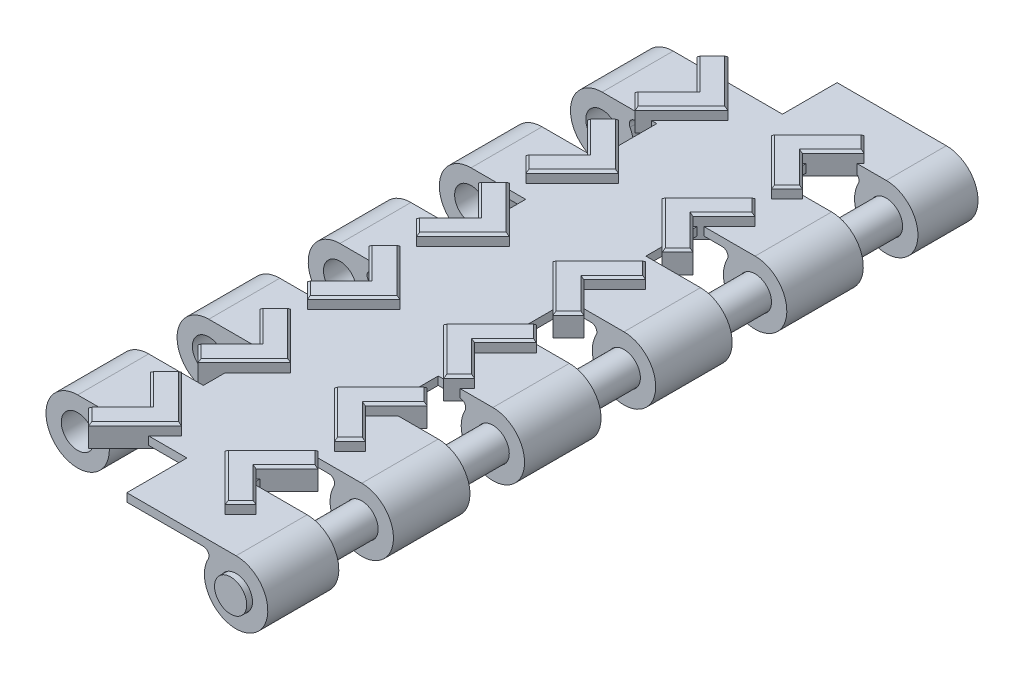
from build123d import *

# Parameters (mm, degrees)
BOSS_EXTRUDE1_DEPTH = 65
SKETCH2_W           = 12.9
SKETCH2_H           = 5.5
SKETCH2_H_2         = 5
CUT_EXTRUDE1_DEPTH  = 78.518380207
BOSS_EXTRUDE2_START = 5
SKETCH3_6_W         = 5
SKETCH3_6_H         = 0.75
BOSS_EXTRUDE2_DEPTH = 48
BOSS_EXTRUDE3_START = 32.5
BOSS_EXTRUDE3_DEPTH = 7.5
SKETCH6_R           = 1.5
CUT_EXTRUDE2_DEPTH  = 78.518380207
BOSS_EXTRUDE5_REACH = 79.518
SKETCH_3_6_W        = 5
SKETCH_3_6_H        = 0.75
SKETCH10_R          = 1.475
BOSS_EXTRUDE6_DEPTH = 33
BOSS_EXTRUDE9_DEPTH = 1
CHAMFER3_SIZE       = 0.2


with BuildPart() as part:
    # Sketch1 → Boss-Extrude1 (new body)
    with BuildSketch(Plane.XY):
        with BuildLine():
            Line((10, 40.220508076), (-10, 40.220508076))
            ThreePointArc((-10, 40.220508076), (-12.511473671, 38.770508076), (-12.511473671, 35.870508076))
            Line((-12.511473671, 35.870508076), (-10, 37.320508076))
            Line((-10, 37.320508076), (-7.1, 37.320508076))
            ThreePointArc((-7.1, 37.320508076), (-7.189694081, 38.036176043), (-7.453228027, 38.70757423))
            ThreePointArc((-7.453228027, 38.70757423), (-7.443701391, 39.218003951), (-7, 39.470508076))
            Line((-7, 39.470508076), (7, 39.470508076))
            ThreePointArc((7, 39.470508076), (7.443701391, 39.218003951), (7.453228027, 38.70757423))
            ThreePointArc((7.453228027, 38.70757423), (7.189694081, 38.036176043), (7.1, 37.320508076))
            Line((7.1, 37.320508076), (10, 37.320508076))
            Line((10, 37.320508076), (12.511473671, 35.870508076))
            ThreePointArc((12.511473671, 35.870508076), (12.511473671, 38.770508076), (10, 40.220508076))
        make_face()
        with BuildLine():
            ThreePointArc((7.1, 37.320508076), (9.249424769, 34.519323179), (12.511473671, 35.870508076))
            Line((12.511473671, 35.870508076), (10, 37.320508076))
            Line((10, 37.320508076), (7.1, 37.320508076))
        make_face()
        with BuildLine():
            Line((-10, 37.320508076), (-12.511473671, 35.870508076))
            ThreePointArc((-12.511473671, 35.870508076), (-9.249424769, 34.519323179), (-7.1, 37.320508076))
            Line((-7.1, 37.320508076), (-10, 37.320508076))
        make_face()
    extrude(amount=BOSS_EXTRUDE1_DEPTH)

    # Sketch2 → Cut-Extrude1 (cut, through all)
    with BuildSketch(Plane(origin=(0, 0, 0), x_dir=(1, 0, 0), z_dir=(0, 1, 0))):
        with Locations((-6.45, -50.25)):
            Rectangle(SKETCH2_W, SKETCH2_H)
        with Locations((-6.45, -62.25)):
            Rectangle(SKETCH2_W, SKETCH2_H)
        with Locations((-6.45, -38.25)):
            Rectangle(SKETCH2_W, SKETCH2_H)
        with Locations((-6.45, -26.25)):
            Rectangle(SKETCH2_W, SKETCH2_H)
        with Locations((-6.45, -14.25)):
            Rectangle(SKETCH2_W, SKETCH2_H)
        with Locations((-6.45, -2.25)):
            Rectangle(SKETCH2_W, SKETCH2_H)
        with Locations((6.45, -44)):
            Rectangle(SKETCH2_W, SKETCH2_H_2)
        with Locations((6.45, -56)):
            Rectangle(SKETCH2_W, SKETCH2_H_2)
        with Locations((6.45, -32)):
            Rectangle(SKETCH2_W, SKETCH2_H_2)
        with Locations((6.45, -20)):
            Rectangle(SKETCH2_W, SKETCH2_H_2)
        with Locations((6.45, -8)):
            Rectangle(SKETCH2_W, SKETCH2_H_2)
    extrude(amount=CUT_EXTRUDE1_DEPTH, mode=Mode.SUBTRACT)

    # Sketch3<6> → Boss-Extrude2 (add)
    with BuildSketch(Plane.XY.offset(BOSS_EXTRUDE2_START)):
        with Locations((-2.5, 39.845508076)):
            Rectangle(SKETCH3_6_W, SKETCH3_6_H)
    extrude(amount=BOSS_EXTRUDE2_DEPTH)

    # Sketch5 → Boss-Extrude3 (add, symmetric)
    with BuildSketch(Plane.XY.offset(BOSS_EXTRUDE3_START)):
        Polygon((-4, 39.470508076), (4, 39.470508076), (1.5, 36.470508076), (-1.5, 36.470508076), align=None)
    extrude(amount=BOSS_EXTRUDE3_DEPTH, both=True)

    # Sketch6 → Cut-Extrude2 (cut, through all)
    with BuildSketch(Plane(origin=(0, 0, 0), x_dir=(-1, 0, 0), z_dir=(0, 0, -1))):
        with Locations((-10, 37.320508076)):
            Circle(SKETCH6_R)
        with Locations((10, 37.320508076)):
            Circle(SKETCH6_R)
    extrude(amount=-CUT_EXTRUDE2_DEPTH, mode=Mode.SUBTRACT)

    # Boss-Extrude5: up to this face of the body (flat: up to its plane)
    boss_extrude5_end = Plane(part.part.faces().sort_by_distance((8.570145796, 37.969067426, 58.5))[0])
    # 草图3<6> → Boss-Extrude5 (add, up to the picked face)
    with BuildSketch(Plane.XY, mode=Mode.PRIVATE) as boss_extrude5_sk1:
        with Locations((2.5, 39.845508076)):
            Rectangle(SKETCH_3_6_W, SKETCH_3_6_H)
    boss_extrude5_tool1 = split(extrude(boss_extrude5_sk1.sketch, amount=BOSS_EXTRUDE5_REACH, mode=Mode.PRIVATE), bisect_by=boss_extrude5_end, keep=Keep.BOTH, mode=Mode.PRIVATE)
    add(boss_extrude5_tool1.solids().sort_by(Axis((2.5, 39.845508, 0), (0, 0, 1)))[0])

    # Sketch12 → Boss-Extrude9 (add, symmetric)
    with BuildSketch(Plane(origin=(0, 40.220508076, 0), x_dir=(1, 0, 0), z_dir=(0, 1, 0))):
        Polygon((-6.242640687, -3.757359313), (-2, -8), (-6.242640687, -12.242640687), (-7.656854249, -10.828427125), (-4.828427125, -8), (-7.656854249, -5.171572875), align=None)
        Polygon((-6.242640687, -13.757359313), (-2, -18), (-6.242640687, -22.242640687), (-7.656854249, -20.828427125), (-4.828427125, -18), (-7.656854249, -15.171572875), align=None)
        Polygon((-6.242640687, -23.757359313), (-2, -28), (-6.242640687, -32.242640687), (-7.656854249, -30.828427125), (-4.828427125, -28), (-7.656854249, -25.171572875), align=None)
        Polygon((-6.242640687, -33.757359313), (-2, -38), (-6.242640687, -42.242640687), (-7.656854249, -40.828427125), (-4.828427125, -38), (-7.656854249, -35.171572875), align=None)
        Polygon((-6.242640687, -43.757359313), (-2, -48), (-6.242640687, -52.242640687), (-7.656854249, -50.828427125), (-4.828427125, -48), (-7.656854249, -45.171572875), align=None)
        Polygon((-6.242640687, -53.757359313), (-2, -58), (-6.242640687, -62.242640687), (-7.656854249, -60.828427125), (-4.828427125, -58), (-7.656854249, -55.171572875), align=None)
        Polygon((4.828427125, -58), (7.656854249, -55.171572875), (6.242640687, -53.757359313), (2, -58), (6.242640687, -62.242640687), (7.656854249, -60.828427125), align=None)
        Polygon((2, -48), (6.242640687, -52.242640687), (7.656854249, -50.828427125), (4.828427125, -48), (7.656854249, -45.171572875), (6.242640687, -43.757359313), align=None)
        Polygon((2, -38), (6.242640687, -42.242640687), (7.656854249, -40.828427125), (4.828427125, -38), (7.656854249, -35.171572875), (6.242640687, -33.757359313), align=None)
        Polygon((2, -28), (6.242640687, -32.242640687), (7.656854249, -30.828427125), (4.828427125, -28), (7.656854249, -25.171572875), (6.242640687, -23.757359313), align=None)
        Polygon((7.656854249, -20.828427125), (4.828427125, -18), (7.656854249, -15.171572875), (6.242640687, -13.757359313), (2, -18), (6.242640687, -22.242640687), align=None)
        Polygon((7.656854249, -5.171572875), (6.242640687, -3.757359313), (2, -8), (6.242640687, -12.242640687), (7.656854249, -10.828427125), (4.828427125, -8), align=None)
    extrude(amount=BOSS_EXTRUDE9_DEPTH, both=True)

    # Chamfer3
    chamfer3_edges = [part.edges().sort_by_distance(p)[0] for p in [
        (4.121320344, 41.220508076, 35.878679656),
        (4.121320344, 41.220508076, 40.121320344),
        (6.949747468, 41.220508076, 41.535533906),
        (6.242640687, 41.220508076, 39.414213562),
        (6.242640687, 41.220508076, 36.585786438),
        (6.949747468, 41.220508076, 34.464466094),
        (4.121320344, 41.220508076, 45.878679656),
        (4.121320344, 41.220508076, 50.121320344),
        (6.949747468, 41.220508076, 51.535533906),
        (6.242640687, 41.220508076, 49.414213562),
        (6.242640687, 41.220508076, 46.585786438),
        (6.949747468, 41.220508076, 44.464466094),
        (-6.949747468, 41.220508076, 54.464466094),
        (-6.242640687, 41.220508076, 56.585786438),
        (-6.242640687, 41.220508076, 59.414213562),
        (-6.949747468, 41.220508076, 61.535533906),
        (-4.121320344, 41.220508076, 60.121320344),
        (-4.121320344, 41.220508076, 55.878679656),
        (-6.949747468, 41.220508076, 44.464466094),
        (-6.242640687, 41.220508076, 46.585786438),
        (-6.242640687, 41.220508076, 49.414213562),
        (-6.949747468, 41.220508076, 51.535533906),
        (-4.121320344, 41.220508076, 50.121320344),
        (-4.121320344, 41.220508076, 45.878679656),
        (-6.949747468, 41.220508076, 34.464466094),
        (-6.242640687, 41.220508076, 36.585786438),
        (-6.242640687, 41.220508076, 39.414213562),
        (-6.949747468, 41.220508076, 41.535533906),
        (-4.121320344, 41.220508076, 40.121320344),
        (-4.121320344, 41.220508076, 35.878679656),
        (-6.949747468, 41.220508076, 24.464466094),
        (-6.242640687, 41.220508076, 26.585786438),
        (-6.242640687, 41.220508076, 29.414213562),
        (-6.949747468, 41.220508076, 31.535533906),
        (-4.121320344, 41.220508076, 30.121320344),
        (-4.121320344, 41.220508076, 25.878679656),
        (-6.949747468, 41.220508076, 14.464466094),
        (-6.242640687, 41.220508076, 16.585786438),
        (-6.242640687, 41.220508076, 19.414213562),
        (-6.949747468, 41.220508076, 21.535533906),
        (-4.121320344, 41.220508076, 20.121320344),
        (-4.121320344, 41.220508076, 15.878679656),
        (-6.949747468, 41.220508076, 4.464466094),
        (-6.242640687, 41.220508076, 6.585786438),
        (-6.242640687, 41.220508076, 9.414213562),
        (-6.949747468, 41.220508076, 11.535533906),
        (-4.121320344, 41.220508076, 10.121320344),
        (-4.121320344, 41.220508076, 5.878679656),
        (4.121320344, 41.220508076, 25.878679656),
        (4.121320344, 41.220508076, 30.121320344),
        (6.949747468, 41.220508076, 31.535533906),
        (6.242640687, 41.220508076, 29.414213562),
        (6.242640687, 41.220508076, 26.585786438),
        (6.949747468, 41.220508076, 24.464466094),
        (6.949747468, 41.220508076, 21.535533906),
        (6.242640687, 41.220508076, 19.414213562),
        (6.242640687, 41.220508076, 16.585786438),
        (6.949747468, 41.220508076, 14.464466094),
        (4.121320344, 41.220508076, 15.878679656),
        (4.121320344, 41.220508076, 20.121320344),
        (6.242640687, 41.220508076, 6.585786438),
        (6.949747468, 41.220508076, 4.464466094),
        (4.121320344, 41.220508076, 5.878679656),
        (4.121320344, 41.220508076, 10.121320344),
        (6.949747468, 41.220508076, 11.535533906),
        (6.242640687, 41.220508076, 9.414213562),
        (6.242640687, 41.220508076, 59.414213562),
        (6.242640687, 41.220508076, 56.585786438),
        (6.949747468, 41.220508076, 54.464466094),
        (4.121320344, 41.220508076, 55.878679656),
        (4.121320344, 41.220508076, 60.121320344),
        (6.949747468, 41.220508076, 61.535533906),
    ]]
    chamfer(chamfer3_edges, length=CHAMFER3_SIZE)


with BuildPart() as body_2:
    # Sketch10 → Boss-Extrude6 (new, symmetric)
    with BuildSketch(Plane(origin=(0, 0, 32.5), x_dir=(-1, 0, 0), z_dir=(0, 0, -1))):
        with Locations((-10, 37.320508076)):
            Circle(SKETCH10_R)
    extrude(amount=BOSS_EXTRUDE6_DEPTH, both=True)


solid = Compound([part.part, body_2.part])
